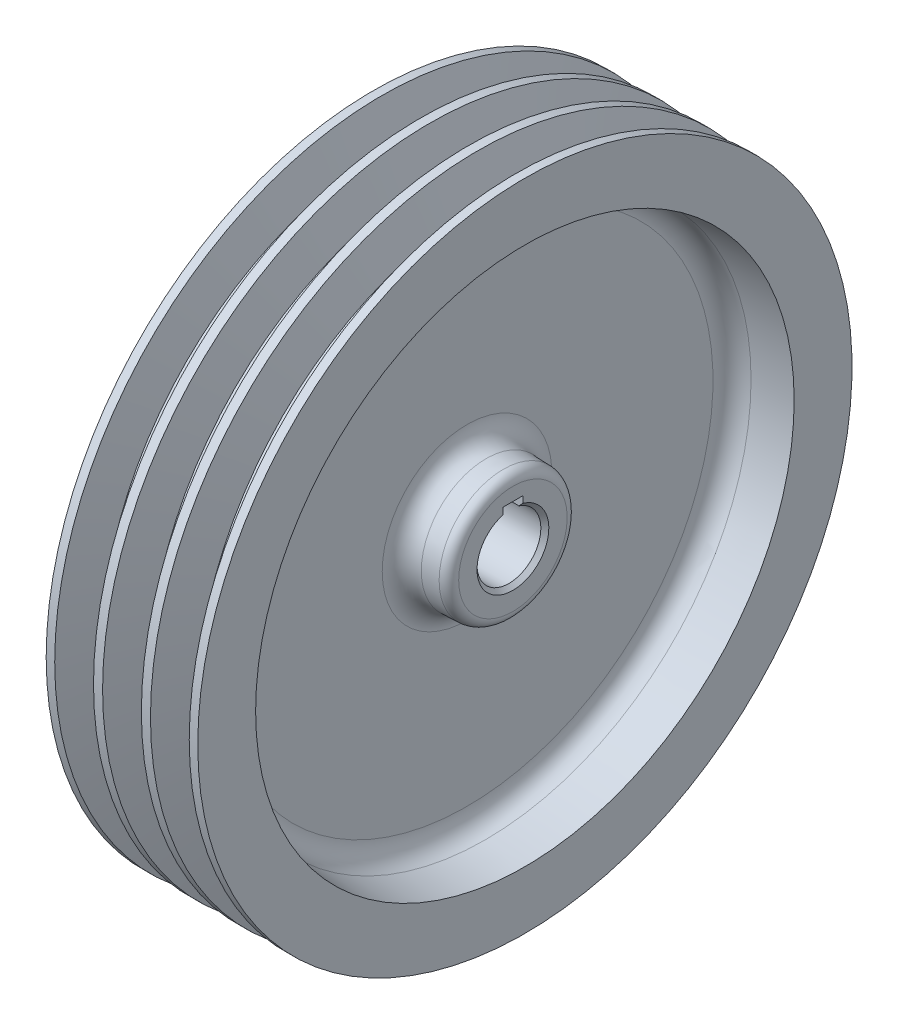
from build123d import *

# Parameters (mm, degrees)
PATTERN_LINEAR_940_COUNT = 3
PATTERN_LINEAR_940_PITCH = 12
CHAMFER_1_SIZE           = 1
SKETCH_4_W               = 5
SKETCH_4_H               = 2.700657875
CUT_EXTRUDE_1_DEPTH      = 122.132159231
FILLET_1_R               = 5
FILLET_2_R               = 2.5


with BuildPart() as part:
    # 草图1 → 旋转1 (revolve)
    with BuildSketch(Plane.XY, mode=Mode.PRIVATE) as revolve_1_sk:
        Polygon((3, 8), (3, 16), (14.5, 17.006119631), (14.5, 66.920154632), (0, 67.5), (0, 82), (38, 82), (38, 67.5), (23.5, 66.231414379), (23.5, 16.459877361), (35, 16), (35, 8), align=None)
    revolve(revolve_1_sk.sketch.rotate(Axis((0, 0, 0), (1, 0, 0)), 90), axis=Axis((0, 0, 0), (1, 0, 0)))

    # 草图2 → 切除-旋转1 (revolve, cut)
    with BuildSketch(Plane.XY, mode=Mode.PRIVATE) as cut_revolve_1_sk:
        Polygon((9.10988523, 73), (11.861461363, 82), (2.138538637, 82), (4.89011477, 73), align=None)
    cut_revolve_1 = revolve(cut_revolve_1_sk.sketch.rotate(Axis((0, 0, 0), (1, 0, 0)), 90), axis=Axis((0, 0, 0), (1, 0, 0)), mode=Mode.SUBTRACT)

    # Pattern Linear 940: 切除-旋转1 ×3
    with Locations(*[(i * PATTERN_LINEAR_940_PITCH, 0, 0) for i in range(1, PATTERN_LINEAR_940_COUNT)]):
        add(cut_revolve_1, mode=Mode.SUBTRACT)

    # 倒角1
    chamfer_1_edges = [part.edges().sort_by_distance(p)[0] for p in [
        (3, 0, -8),
        (35, 0, -8),
    ]]
    chamfer(chamfer_1_edges, length=CHAMFER_1_SIZE)

    # 草图4 → 切除-拉伸1 (cut, through all)
    with BuildSketch(Plane.ZY.offset(-3)):
        with Locations((0, 8.949671014)):
            Rectangle(SKETCH_4_W, SKETCH_4_H)
    extrude(amount=-CUT_EXTRUDE_1_DEPTH, mode=Mode.SUBTRACT)

    # 圆角1
    fillet_1_edges = [part.edges().sort_by_distance(p)[0] for p in [
        (14.5, 0, -66.920154632),
        (14.5, 0, -17.006119631),
        (23.5, 0, -16.459877361),
        (23.5, 0, -66.231414379),
    ]]
    fillet(fillet_1_edges, radius=FILLET_1_R)

    # 圆角2
    fillet_2_edges = [part.edges().sort_by_distance(p)[0] for p in [
        (3, 0, -16),
        (35, 0, -16),
    ]]
    fillet(fillet_2_edges, radius=FILLET_2_R)


solid = part.part
